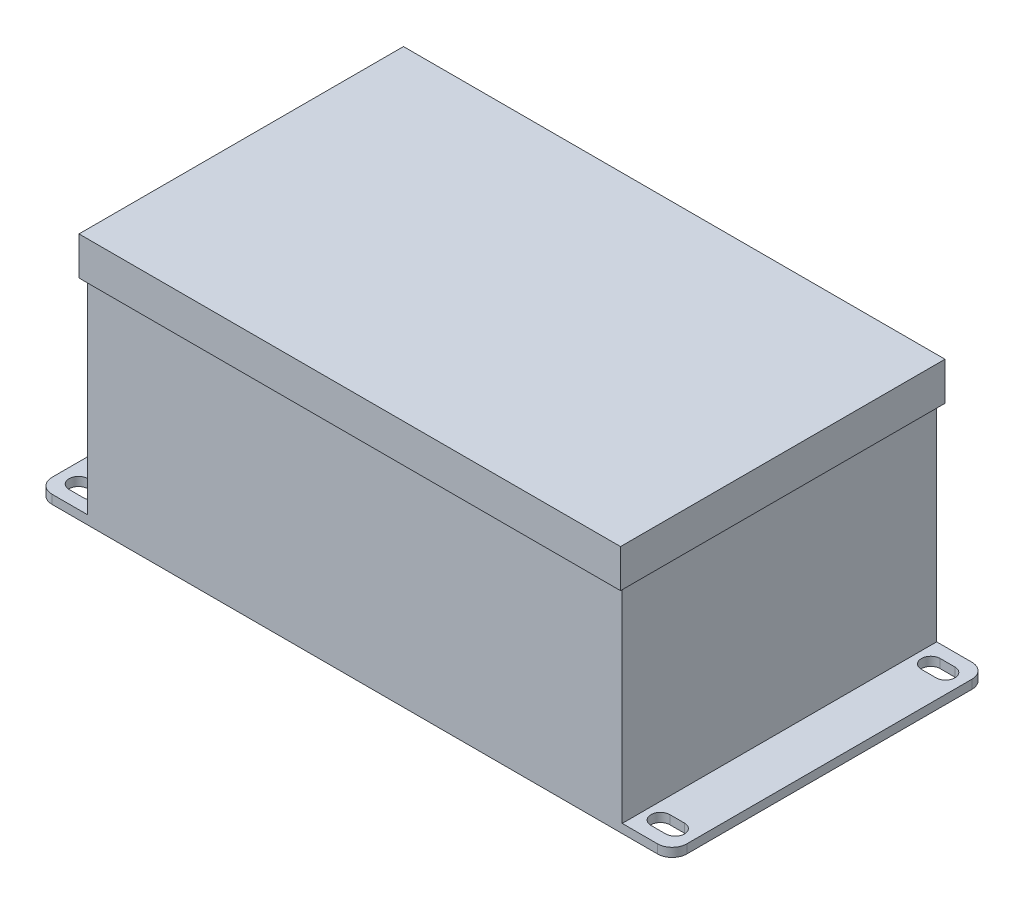
SolidWorks part; units mm, degrees
ref_plane "Front Plane" through (0, 0, 0) normal (0, 0, 1) x (1, 0, 0)
ref_plane "Top Plane" through (0, 0, 0) normal (0, 1, 0) x (1, 0, 0)
ref_plane "Right Plane" through (0, 0, 0) normal (1, 0, 0) x (0, 0, -1)
sketch "Sketch1" plane through (0, 0, 0) normal (0, 1, 0) x (1, 0, 0)
  line L0 (-101.5, 46) -> (-96.5, 46) construction
  line L1 (-103, -53.5) -> (103, -53.5)
  line L2 (-108, -48.5) -> (-108, 48.5)
  line L3 (-103, 53.5) -> (103, 53.5)
  line L4 (108, -48.5) -> (108, 48.5)
  line L5 (-108, -53.5) -> (108, 53.5) construction
  line L6 (-108, 53.5) -> (108, -53.5) construction
  line L7 (-101.5, 49.2) -> (-96.5, 49.2)
  line L8 (-101.5, 42.8) -> (-96.5, 42.8)
  line L9 (96.5, 46) -> (101.5, 46) construction
  line L10 (96.5, 49.2) -> (101.5, 49.2)
  line L11 (96.5, 42.8) -> (101.5, 42.8)
  line L12 (-101.5, -46) -> (-96.5, -46) construction
  line L13 (-101.5, -42.8) -> (-96.5, -42.8)
  line L14 (-101.5, -49.2) -> (-96.5, -49.2)
  line L15 (96.5, -46) -> (101.5, -46) construction
  line L16 (96.5, -42.8) -> (101.5, -42.8)
  line L17 (96.5, -49.2) -> (101.5, -49.2)
  arc A0 (-101.5, 49.2) -> (-101.5, 42.8) centre (-101.5, 46) ccw
  arc A1 (-96.5, 42.8) -> (-96.5, 49.2) centre (-96.5, 46) ccw
  arc A2 (96.5, 49.2) -> (96.5, 42.8) centre (96.5, 46) ccw
  arc A3 (101.5, 42.8) -> (101.5, 49.2) centre (101.5, 46) ccw
  arc A4 (-101.5, -42.8) -> (-101.5, -49.2) centre (-101.5, -46) ccw
  arc A5 (-96.5, -49.2) -> (-96.5, -42.8) centre (-96.5, -46) ccw
  arc A6 (96.5, -42.8) -> (96.5, -49.2) centre (96.5, -46) ccw
  arc A7 (101.5, -49.2) -> (101.5, -42.8) centre (101.5, -46) ccw
  arc A8 (-103, -53.5) -> (-108, -48.5) centre (-103, -48.5) cw
  arc A9 (103, -53.5) -> (108, -48.5) centre (103, -48.5) ccw
  arc A10 (103, 53.5) -> (108, 48.5) centre (103, 48.5) cw
  arc A11 (-108, 48.5) -> (-103, 53.5) centre (-103, 48.5) cw
  point P0 (0, 0)
  point P8 (-99, 46)
  point P13 (99, 46)
  point P20 (-99, -46)
  point P27 (99, -46)
  dimension "D3" = 3.2
  dimension "D4" = 3.2
  dimension "D5" = 3.2
  dimension "D6" = 3.2
  dimension "D19" = 5
  dimension "D1" = 216
  dimension "D2" = 107
  dimension "D7" = 5
  dimension "D8" = 5
  dimension "D9" = 5
  dimension "D10" = 5
  dimension "D11" = 92
  dimension "D12" = 46
  dimension "D13" = 92
  dimension "D14" = 46
  dimension "D15" = 198
  dimension "D16" = 99
  dimension "D17" = 99
  dimension "D18" = 99
extrude "Boss-Extrude1" add sketch "Sketch1" along normal blind 3
sketch "Sketch2" plane through (0, 3, 0) normal (0, 1, 0) x (1, 0, 0)
  line L0 (103, 53.5) -> (-103, 53.5) construction
  line L1 (-91, -53.5) -> (91, -53.5)
  line L2 (-91, -53.5) -> (-91, 53.5)
  line L3 (-91, 53.5) -> (91, 53.5)
  line L4 (91, -53.5) -> (91, 53.5)
  line L5 (-91, -53.5) -> (91, 53.5) construction
  line L6 (-91, 53.5) -> (91, -53.5) construction
  point P0 (0, 0)
  dimension "D1" = 182
extrude "Boss-Extrude2" add sketch "Sketch2" along normal blind 70
sketch "Sketch4" plane through (0, 73, 0) normal (0, 1, 0) x (1, 0, 0)
  line L1 (-92.1309, -55.2057) -> (92.1309, -55.2057)
  line L2 (-92.1309, -55.2057) -> (-92.1309, 55.2057)
  line L3 (-92.1309, 55.2057) -> (92.1309, 55.2057)
  line L4 (92.1309, -55.2057) -> (92.1309, 55.2057)
  line L5 (-92.1309, -55.2057) -> (92.1309, 55.2057) construction
  line L6 (-92.1309, 55.2057) -> (92.1309, -55.2057) construction
  point P0 (0, 0)
extrude "Boss-Extrude3" add sketch "Sketch4" along normal blind 13
